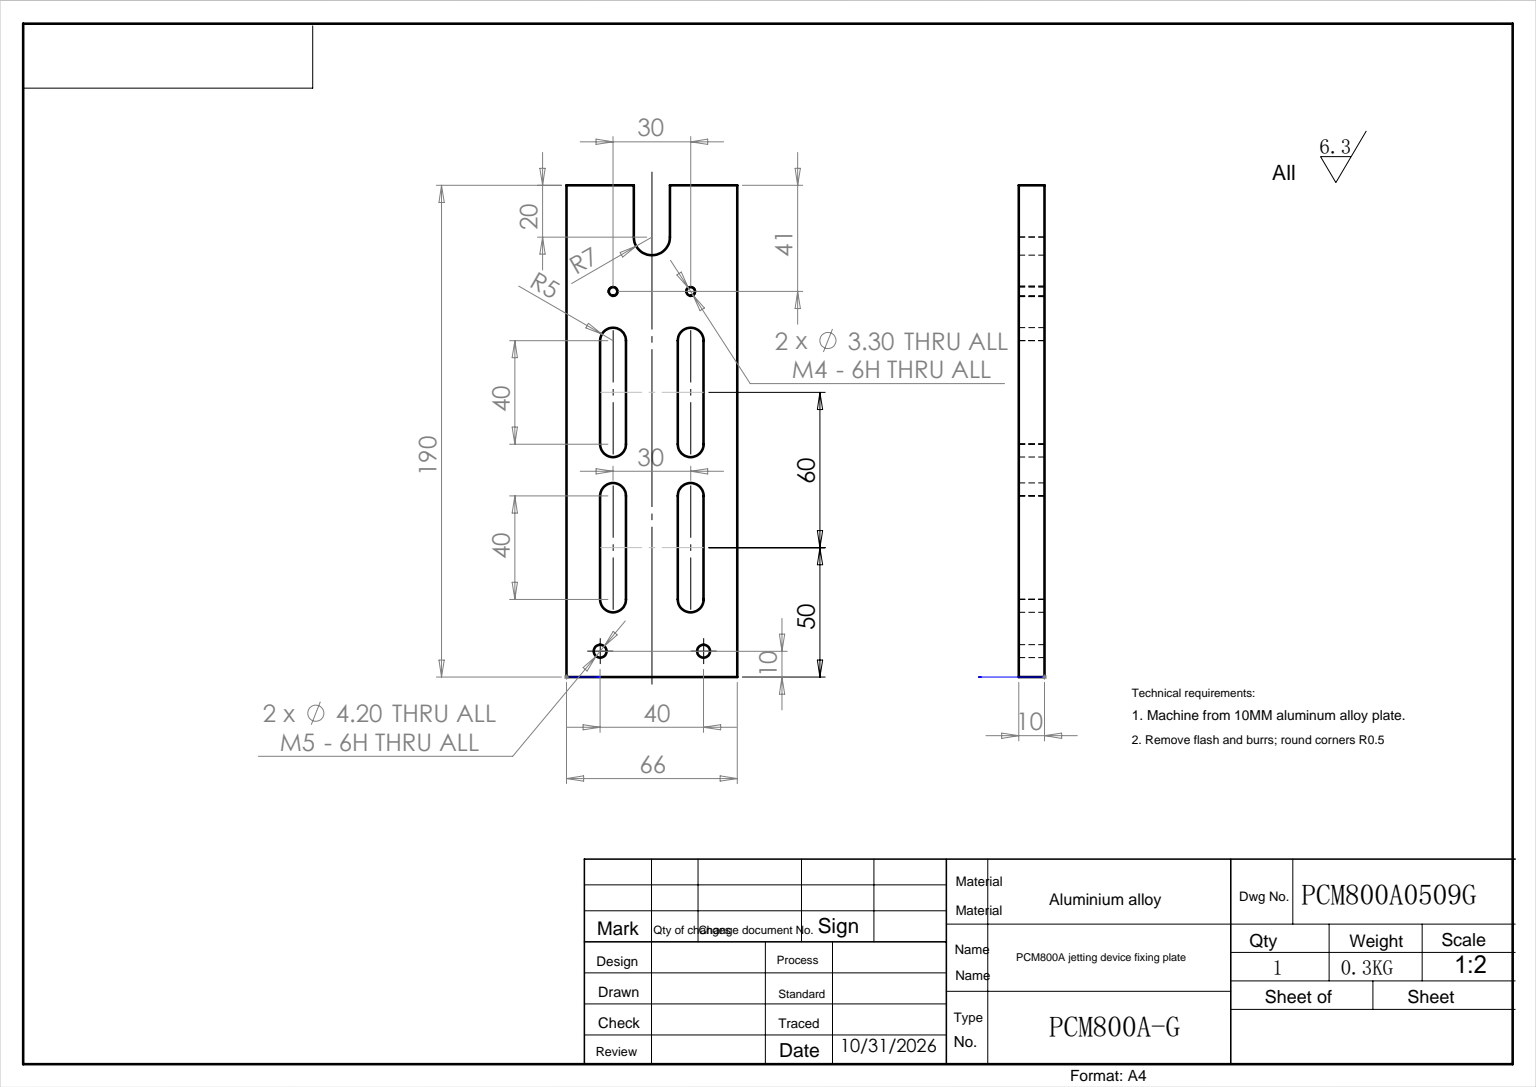
from build123d import *

# Parameters (mm, degrees)
SKETCH_1_W          = 66
SKETCH_1_H          = 10
EXTRUDE_1_DEPTH     = 190
CUT_EXTRUDE_2_DEPTH = 202.385203031
HOLE_WIZARD_M5_1_D  = 5
CUT_EXTRUDE_3_DEPTH = 202.385203031
HOLE_WIZARD_M4_1_D  = 3.3


with BuildPart() as part:
    # 草图1 → 拉伸1 (new body)
    with BuildSketch(Plane.XY):
        with Locations((33, 5)):
            Rectangle(SKETCH_1_W, SKETCH_1_H)
    extrude(amount=EXTRUDE_1_DEPTH)

    # 草图5 → 切除-拉伸2 (cut, through all)
    with BuildSketch(Plane(origin=(0, 10, 0), x_dir=(-1, 0, 0), z_dir=(0, 1, 0))):
        with BuildLine():
            Line((-43, 70), (-43, 30))
            ThreePointArc((-43, 30), (-48, 25), (-53, 30))
            Line((-53, 30), (-53, 70))
            ThreePointArc((-53, 70), (-48, 75), (-43, 70))
        make_face()
        with BuildLine():
            Line((-13, 70), (-13, 30))
            ThreePointArc((-13, 30), (-18, 25), (-23, 30))
            Line((-23, 30), (-23, 70))
            ThreePointArc((-23, 70), (-18, 75), (-13, 70))
        make_face()
        with BuildLine():
            Line((-43, 130), (-43, 90))
            ThreePointArc((-43, 90), (-48, 85), (-53, 90))
            Line((-53, 90), (-53, 130))
            ThreePointArc((-53, 130), (-48, 135), (-43, 130))
        make_face()
        with BuildLine():
            Line((-13, 130), (-13, 90))
            ThreePointArc((-13, 90), (-18, 85), (-23, 90))
            Line((-23, 90), (-23, 130))
            ThreePointArc((-23, 130), (-18, 135), (-13, 130))
        make_face()
    extrude(amount=-CUT_EXTRUDE_2_DEPTH, mode=Mode.SUBTRACT)

    # M5 螺纹孔1 (through all)
    with Locations(Plane(origin=(0, 10, 0), x_dir=(-1, 0, 0), z_dir=(0, 1, 0))):
        with Locations((-13, 10), (-53, 10)):
            Hole(HOLE_WIZARD_M5_1_D / 2)

    # 草图11 → 切除-拉伸3 (cut, through all)
    with BuildSketch(Plane(origin=(0, 10, 0), x_dir=(-1, 0, 0), z_dir=(0, 1, 0))):
        with BuildLine():
            Line((-40, 249.750844229), (-40, 170))
            ThreePointArc((-40, 170), (-33, 163), (-26, 170))
            Line((-26, 170), (-26, 249.750844229))
            Line((-26, 249.750844229), (-40, 249.750844229))
        make_face()
    extrude(amount=-CUT_EXTRUDE_3_DEPTH, mode=Mode.SUBTRACT)

    # M4 螺纹孔1 (through all)
    with Locations(Plane.XZ):
        with Locations((18, 149), (48, 149)):
            Hole(HOLE_WIZARD_M4_1_D / 2)


solid = part.part
